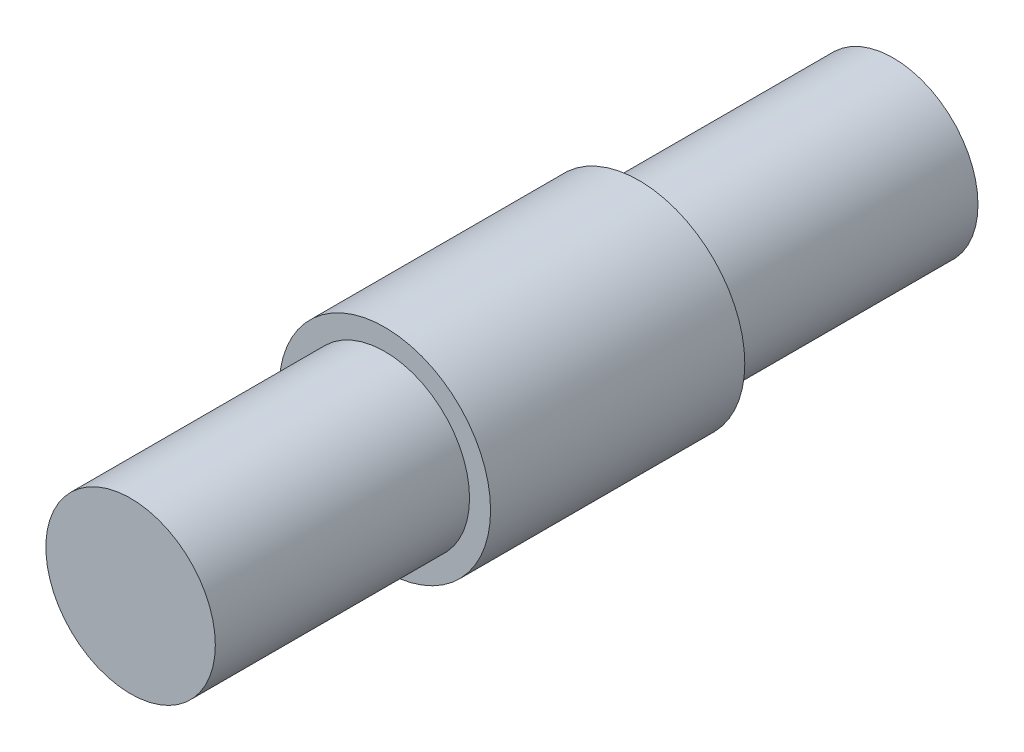
from build123d import *

# Parameters (mm, degrees)
BOSS_EXTRUDE1_DEPTH      = 4.7625
BOSS_EXTRUDE1_DEPTH_BACK = 4.7625
SKETCH1_R                = 3.9624
BOSS_EXTRUDE2_DEPTH      = 14.2875
BOSS_EXTRUDE2_DEPTH_BACK = 14.2875
BOSS_EXTRUDE2_START      = -4.7625
SKETCH2_R                = 3.175


with BuildPart() as part:
    # Sketch1 → Boss-Extrude1 (new, two sides: drawn at the far end of the back side and taken through both)
    with BuildSketch(Plane.XY.offset(-BOSS_EXTRUDE1_DEPTH_BACK)):
        Circle(SKETCH1_R)
    extrude(amount=BOSS_EXTRUDE1_DEPTH + BOSS_EXTRUDE1_DEPTH_BACK)

    # Sketch2 → Boss-Extrude2 (add, two sides: drawn at the far end of the back side and taken through both)
    with BuildSketch(Plane.XY.offset(4.7625).offset(BOSS_EXTRUDE2_START - BOSS_EXTRUDE2_DEPTH_BACK)):
        Circle(SKETCH2_R)
    extrude(amount=BOSS_EXTRUDE2_DEPTH + BOSS_EXTRUDE2_DEPTH_BACK)


solid = part.part
